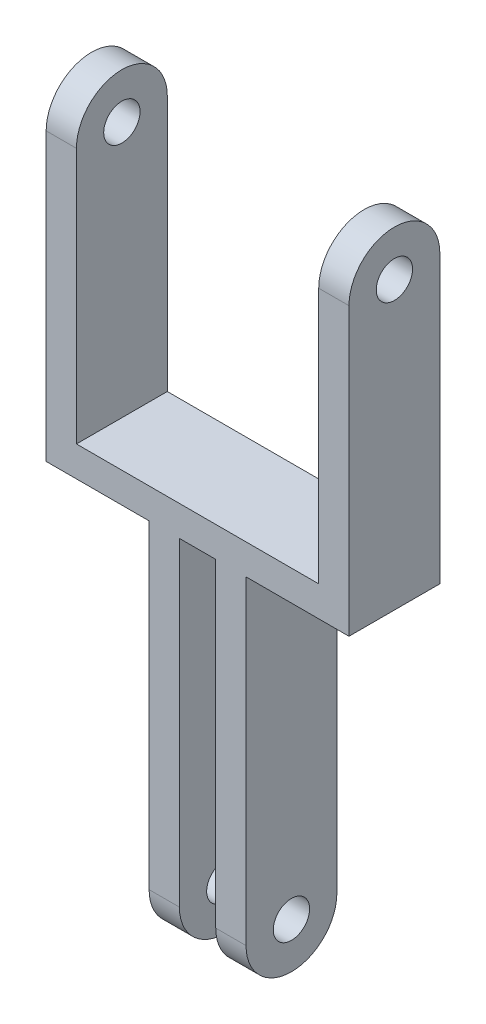
from build123d import *

# Parameters (mm, degrees)
BOSS_EXTRUDE1_DEPTH = 15
SKETCH2_R           = 3
CUT_EXTRUDE1_DEPTH  = 131.862523283


with BuildPart() as part:
    # Sketch1 → Boss-Extrude1 (new body)
    with BuildSketch(Plane.XY):
        Polygon((-3, 0), (-3, 65), (3, 65), (3, 0), (8, 0), (8, 65), (25, 65), (25, 120), (20, 120), (20, 70), (-20, 70), (-20, 120), (-25, 120), (-25, 65), (-8, 65), (-8, 0), align=None)
    extrude(amount=BOSS_EXTRUDE1_DEPTH)

    # Sketch2 → Cut-Extrude1 (cut, through all)
    with BuildSketch(Plane.ZY.offset(25)):
        with Locations(Location((7.5, 112.271855303, 0), (0, 0, 270))):
            Circle(SKETCH2_R)
        with Locations(Location((7.5, 12.271855303, 0), (0, 0, 270))):
            Circle(SKETCH2_R)
        with BuildLine():
            Line((0, 112.271855303), (-22.426817963, 115.88465347))
            Line((-22.426817963, 115.88465347), (0, 149.126440397))
            Line((0, 149.126440397), (35.619754134, 129.721336353))
            Line((35.619754134, 129.721336353), (15, 112.271855303))
            ThreePointArc((15, 112.271855303), (7.5, 119.771855303), (0, 112.271855303))
        make_face()
        with BuildLine():
            Line((0, 12.271855303), (-15.301630232, 4.771855303))
            Line((-15.301630232, 4.771855303), (-3.280552195, -11.427643596))
            Line((-3.280552195, -11.427643596), (32.469088575, -8.187179082))
            Line((32.469088575, -8.187179082), (24.8383173, 8.521855303))
            Line((24.8383173, 8.521855303), (15, 12.271855303))
            ThreePointArc((15, 12.271855303), (7.5, 4.771855303), (0, 12.271855303))
        make_face()
    extrude(amount=-CUT_EXTRUDE1_DEPTH, mode=Mode.SUBTRACT)


solid = part.part
